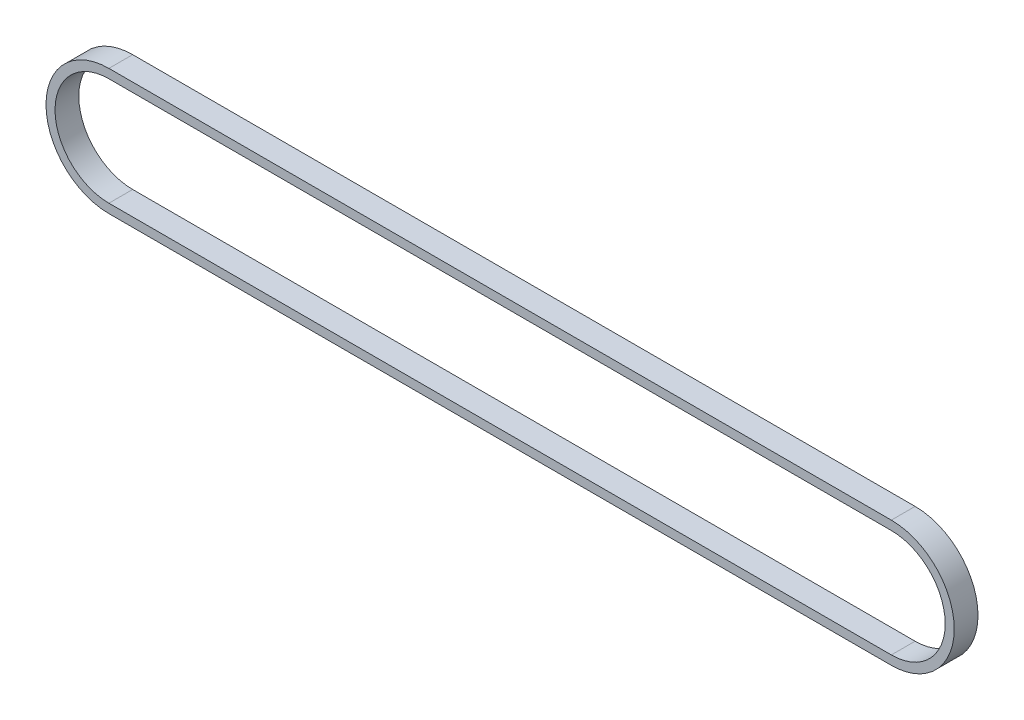
from build123d import *

# Parameters (mm, degrees)
BOSS_EXTRUDE1_DEPTH = 7.9
SHELL1_T            = -3


with BuildPart() as part:
    # Sketch2 → Boss-Extrude1 (new body)
    with BuildSketch(Plane.XY):
        with BuildLine():
            Line((0, 20.9), (-260, 20.9))
            ThreePointArc((-260, 20.9), (-280.9, 0), (-260, -20.9))
            Line((-260, -20.9), (0, -20.9))
            ThreePointArc((0, -20.9), (20.9, 0), (0, 20.9))
        make_face()
    extrude(amount=BOSS_EXTRUDE1_DEPTH)

    # Shell1
    shell1_openings = [part.faces().sort_by_distance(p)[0] for p in [
        (-130, 0, 7.9),
        (-130, 0, 0),
    ]]
    offset(amount=SHELL1_T, openings=shell1_openings, kind=Kind.INTERSECTION)


solid = part.part
